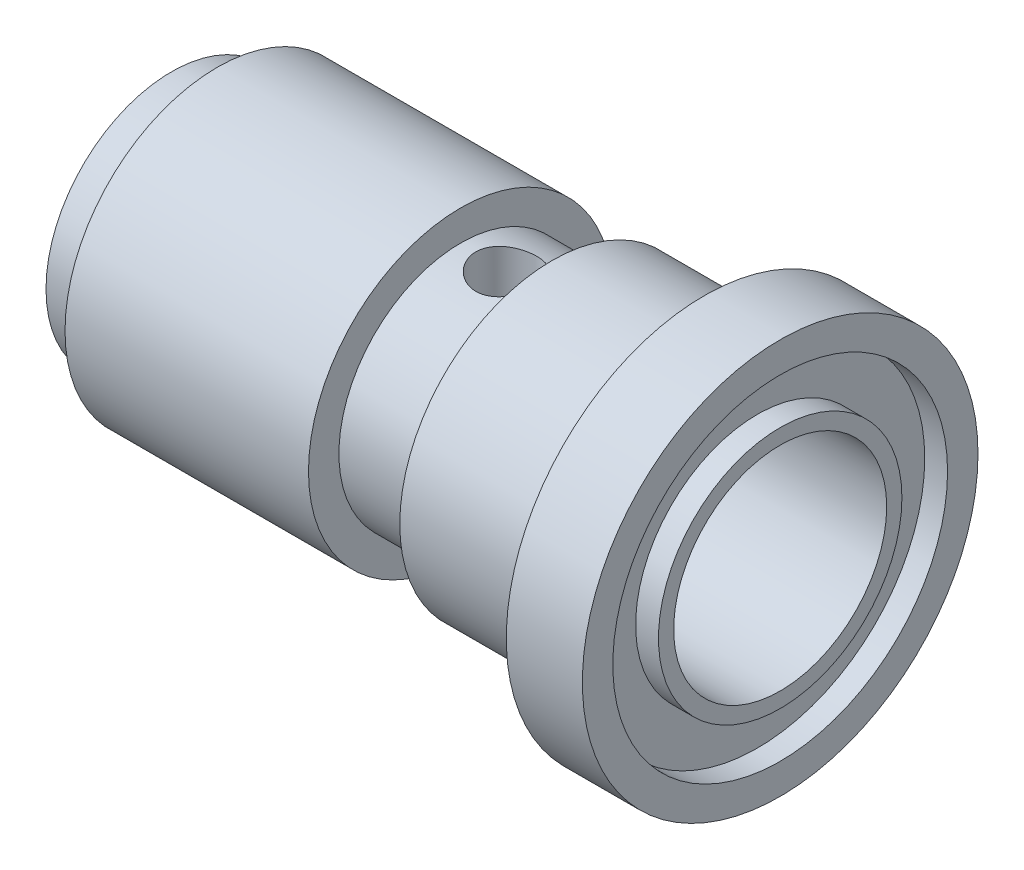
SolidWorks part; units mm, degrees
ref_plane "Front Plane" through (0, 0, 0) normal (0, 0, 1) x (1, 0, 0)
ref_plane "Top Plane" through (0, 0, 0) normal (0, 1, 0) x (1, 0, 0)
ref_plane "Right Plane" through (0, 0, 0) normal (1, 0, 0) x (0, 0, -1)
other "Configuration Table"
sketch "Sketch1" plane through (0, 0, 0) normal (1, 0, 0) x (0, 0, -1)
  circle A0 centre (0, 0) radius 8.25
  dimension "D1" = 16.5
extrude "Boss-Extrude1" add sketch "Sketch1" along normal blind 3
sketch "Sketch2" plane through (3, 0, 0) normal (1, 0, 0) x (0, 0, -1)
  circle A0 centre (0, 0) radius 10
  dimension "D1" = 20
extrude "Boss-Extrude2" add sketch "Sketch2" along normal blind 32
sketch "Sketch4" plane through (35, 0, 0) normal (1, 0, 0) x (0, 0, -1)
  circle A0 centre (0, 0) radius 13
  dimension "D1" = 26
extrude "Boss-Extrude3" add sketch "Sketch4" along normal blind 5
sketch "Sketch5" plane through (40, 0, 0) normal (1, 0, 0) x (0, 0, -1)
  circle A0 centre (0, 0) radius 7
  dimension "D1" = 14
extrude "Cut-Extrude1" cut sketch "Sketch5" against normal blind 10
sketch "Sketch6" plane through (30, 0, 0) normal (1, 0, 0) x (0, 0, -1)
  circle A0 centre (0, 0) radius 2.5
  dimension "D1" = 5
extrude "Cut-Extrude2" cut sketch "Sketch6" against normal blind 33
sketch "Sketch7" plane through (0, 0, 0) normal (-1, 0, 0) x (0, 0, 1)
  circle A0 centre (0, 0) radius 3.75
  dimension "D1" = 7.5
extrude "Cut-Extrude3" cut sketch "Sketch7" against normal blind 6.5
sketch "Sketch8" plane through (0, 0, 0) normal (0, 0, 1) x (1, 0, 0)
  line L0 (22, 11.2682) -> (22, -10.5694)
  line L1 (0, 8.25) -> (0, -8.25) construction
  dimension "D1" = 22
sweep "Cut-Sweep1" cut path "Sketch8" circular profile diameter 4 parameters "D3"=4
sketch "Sketch15" plane through (0, 0, 0) normal (0, 0, 1) x (1, 0, 0)
  line L0 (22, 10.4067) -> (22, 4.8099) construction
  line L1 (0, 8.25) -> (0, -8.25) construction
  line L2 (0, 0) -> (-9.5402, 0) construction
  line L3 (19, 12.8135) -> (25, 12.8135)
  line L4 (19, 12.8135) -> (19, 8)
  line L5 (19, 8) -> (25, 8)
  line L6 (25, 12.8135) -> (25, 8)
  line L7 (19, 12.8135) -> (25, 8) construction
  line L8 (19, 8) -> (25, 12.8135) construction
  dimension "D1" = 22
  dimension "D2" = 8
  dimension "D3" = 6
revolve "Cut-Revolve1" cut sketch "Sketch15" angle 360 about L2
sketch "Sketch17" plane through (40, 0, 0) normal (1, 0, 0) x (0, 0, -1)
  circle A0 centre (0, 0) radius 11
  circle A1 centre (0, 0) radius 8
  dimension "D1" = 22
  dimension "D2" = 16
extrude "Cut-Extrude4" cut sketch "Sketch17" against normal blind 1.5
